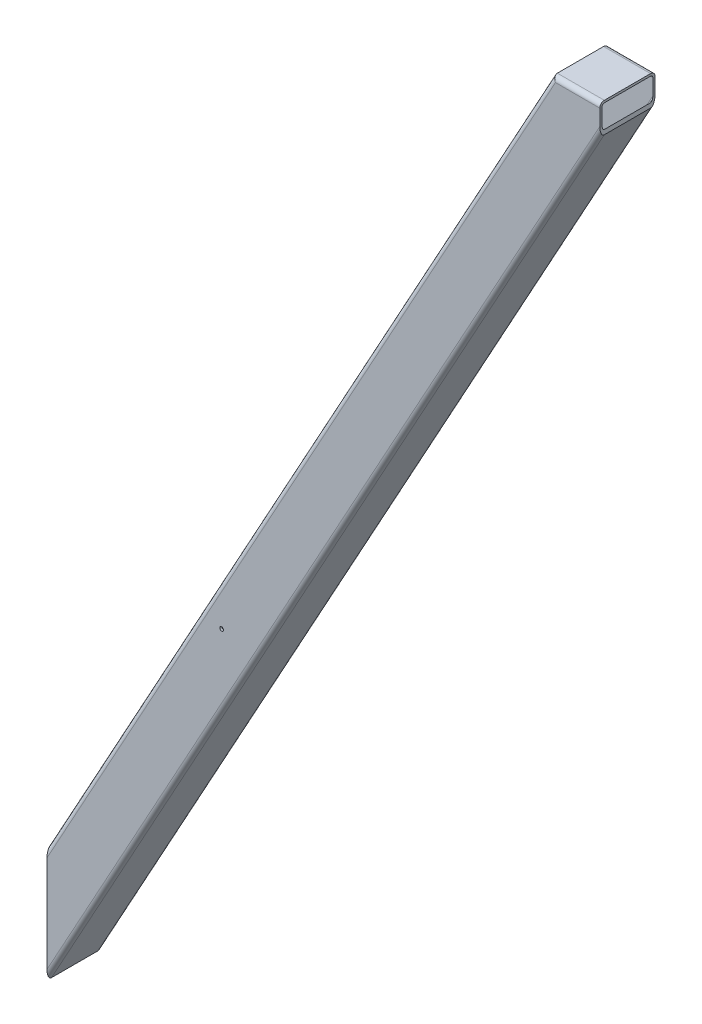
from build123d import *

# Parameters (mm, degrees)
BOSS_EXTRUDE1_DEPTH   = 100
SHELL1_T              = -4
FILLET1_R             = 8.2
FILLET2_R             = 4.2
M8_TAPPED_HOLE1_D     = 6.8
M8_TAPPED_HOLE1_DEPTH = 19.75
M8_TAPPED_HOLE1_TIP   = 2.042926105


with BuildPart() as part:
    # Sketch1 → Boss-Extrude1 (new body)
    with BuildSketch(Plane.XY):
        Polygon((0, 0), (0, 208.736831721), (915, 1874.433314365), (1000, 1874.433314365), (1000, 1820.433314365), align=None)
    extrude(amount=BOSS_EXTRUDE1_DEPTH)

    # Shell1
    shell1_openings = [part.faces().sort_by_distance(p)[0] for p in [
        (0, 104.36841586, 50),
        (1000, 1847.433314365, 50),
    ]]
    offset(amount=SHELL1_T, openings=shell1_openings, kind=Kind.INTERSECTION)

    # Fillet1
    fillet1_edges = [part.edges().sort_by_distance(p)[0] for p in [
        (457.5, 1041.585073043, 100),
        (957.5, 1874.433314365, 100),
        (957.5, 1874.433314365, 0),
        (457.5, 1041.585073043, 0),
        (500, 910.216657182, 0),
        (500, 910.216657182, 100),
    ]]
    fillet(fillet1_edges, radius=FILLET1_R)

    # Fillet2
    fillet2_edges = [part.edges().sort_by_distance(p)[0] for p in [
        (958.683247588, 1870.433314365, 96),
        (458.683247588, 1035.431049715, 96),
        (500, 918.524703838, 96),
        (500, 918.524703838, 4),
        (458.683247588, 1035.431049715, 4),
        (958.683247588, 1870.433314365, 4),
    ]]
    fillet(fillet2_edges, radius=FILLET2_R)

    # M8 Tapped Hole1
    with Locations(Plane.XY.offset(100)):
        with Locations((316, 708.43)):
            Hole(M8_TAPPED_HOLE1_D / 2, depth=M8_TAPPED_HOLE1_DEPTH)
            with Locations((0, 0, -(M8_TAPPED_HOLE1_DEPTH + M8_TAPPED_HOLE1_TIP / 2))):  # 118° drill point
                Cone(0, M8_TAPPED_HOLE1_D / 2, M8_TAPPED_HOLE1_TIP, mode=Mode.SUBTRACT)


solid = part.part
